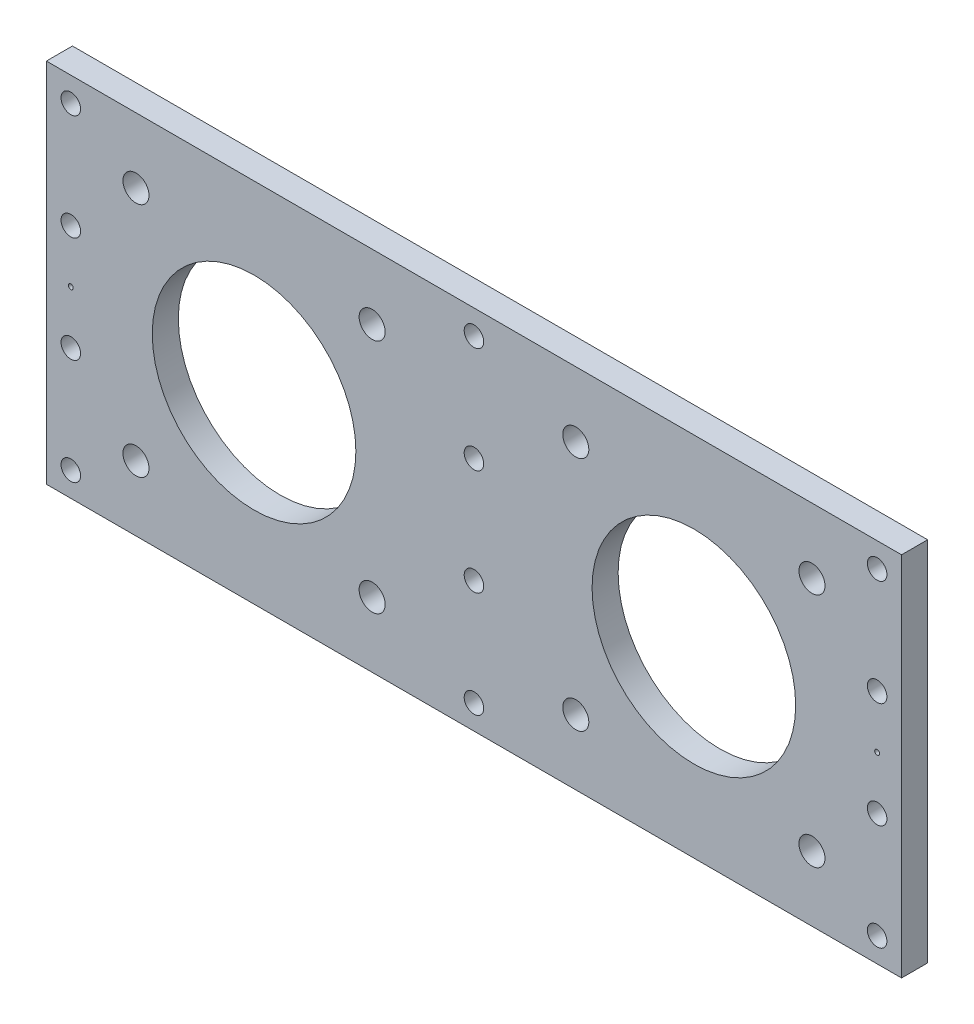
SolidWorks part; units mm, degrees
ref_plane "Front" through (0, 0, 0) normal (0, 0, 1) x (1, 0, 0)
ref_plane "Top" through (0, 0, 0) normal (0, 1, 0) x (1, 0, 0)
ref_plane "Right" through (0, 0, 0) normal (1, 0, 0) x (0, 0, -1)
sketch "Sketch1" plane through (0, 0, 0) normal (0, 0, 1) x (1, 0, 0)
  line L1 (-73.9828, 395.0592) -> (976.0172, 395.0592)
  line L2 (-73.9828, 395.0592) -> (-73.9828, -54.9408)
  line L3 (-73.9828, -54.9408) -> (976.0172, -54.9408)
  line L4 (976.0172, 395.0592) -> (976.0172, -54.9408)
extrude "Boss-Extrude1" add sketch "Sketch1" along normal blind 32
sketch "Sketch2" plane through (0, 0, 32) normal (0, 0, 1) x (1, 0, 0)
  line L0 (451.0172, 395.0592) -> (451.0172, -54.9408) construction
  line L1 (976.0172, 395.0592) -> (-73.9828, 395.0592) construction
  line L2 (-73.9828, -54.9408) -> (976.0172, -54.9408) construction
  line L3 (181.0172, 395.0592) -> (181.0172, -54.9408) construction
  line L4 (-73.9828, 170.0592) -> (976.0172, 170.0592) construction
  line L5 (-73.9828, 395.0592) -> (-73.9828, -54.9408) construction
  line L6 (976.0172, -54.9408) -> (976.0172, 395.0592) construction
  line L7 (721.0172, 395.0592) -> (721.0172, -54.9408) construction
  circle A0 centre (181.0172, 170.0592) radius 125
  circle A1 centre (721.0172, 170.0592) radius 125
  dimension "D2" = 125
  dimension "D3" = 125
  dimension "D1" = 255
extrude "Cut-Extrude1" cut sketch "Sketch2" against normal blind 32
sketch "Sketch3" plane through (0, 0, 32) normal (0, 0, 1) x (1, 0, 0)
  line L0 (976.0172, 395.0592) -> (-73.9828, 395.0592) construction
  line L1 (-73.9828, 395.0592) -> (-73.9828, -54.9408) construction
  line L2 (451.0172, 395.0592) -> (451.0172, -54.9408) construction
  line L3 (-73.9828, -54.9408) -> (976.0172, -54.9408) construction
  circle A0 centre (-43.9828, 365.0592) radius 12
  circle A1 centre (-43.9828, 235.0592) radius 12
  circle A2 centre (-43.9828, 105.0592) radius 12
  circle A3 centre (-43.9828, -24.9408) radius 12
  circle A4 centre (946.0172, -24.9408) radius 12
  circle A5 centre (946.0172, 105.0592) radius 12
  circle A6 centre (946.0172, 235.0592) radius 12
  circle A7 centre (946.0172, 365.0592) radius 12
  circle A8 centre (451.0172, 365.0592) radius 12
  circle A9 centre (451.0172, 235.0592) radius 12
  circle A10 centre (451.0172, 105.0592) radius 12
  circle A11 centre (451.0172, -24.9408) radius 12
  dimension "D1" = 24
  dimension "D2" = 30
  dimension "D3" = 30
  dimension "D5" = 12
  dimension "D4" = 4
  dimension "D6" = 4
extrude "Cut-Extrude2" cut sketch "Sketch3" against normal blind 32
sketch "Sketch4" plane through (0, 0, 32) normal (0, 0, 1) x (1, 0, 0)
  line L0 (181.0172, 295.0592) -> (181.0172, 45.0592) construction
  line L1 (181.0172, 170.0592) -> (36.0603, 315.0161) construction
  line L5 (56.0172, 170.0592) -> (306.0172, 170.0592) construction
  circle A0 centre (181.0172, 170.0592) radius 125 construction
  circle A1 centre (36.0603, 315.0161) radius 18
  circle A2 centre (181.0172, 170.0592) radius 205 construction
  dimension "D5" = 410
  dimension "D1" = 45
hole_wizard "M36 Tapped Hole1" positions "Sketch6" profile "Sketch5" tap size "M36" standard "GB"
sketch "Sketch6" plane through (0, 0, 32) normal (0, 0, 1) x (1, 0, 0)
  line L0 (181.0172, 170.0592) -> (36.0172, 315.0592) construction
  line L2 (181.0172, 170.0592) -> (181.0172, 495.7981) construction
  circle A1 centre (181.0172, 170.0592) radius 205.061 construction
  point P0 (36.0172, 315.0592)
  dimension "D1" = 410.1219
  dimension "D2" = 45
sketch "Sketch5" plane through (36.0172, 315.0592, 32) normal (1, 0, 0) x (0, -1, 0)
  line L0 (0, 0) -> (0, 101.6138)
  line L1 (0, 101.6138) -> (16, 92)
  line L2 (16, 92) -> (16, 0)
  line L5 (16, 0) -> (0, 0)
  line L10 (0, 101.6138) -> (-16, 92) construction
  line L11 (0, -6.35) -> (0, 107.95) construction
  dimension "螺纹孔钻头直径" = 32
  dimension "螺纹孔钻头深度" = 92
  dimension "导头角度" = 118
cosmetic thread "Cosmetic Thread4" parameters "D1"=32, "D2"=36
ref_plane "Plane1" through (451.0172, 0, 0) normal (-1, 0, 0) x (0, 0, 1)
mirror "Mirror1" about plane through (451.0172, 0, 0) normal (-1, 0, 0) of "M36 Tapped Hole1"
sketch "Sketch7" plane through (0, 0, 32) normal (0, 0, 1) x (1, 0, 0)
  line L0 (56.0172, 170.0592) -> (-73.9828, 170.0592) construction
  line L1 (-73.9828, 395.0592) -> (-73.9828, -54.9408) construction
  line L2 (-43.9828, 223.0592) -> (-43.9828, 117.0592) construction
  circle A0 centre (-43.9828, 235.0592) radius 12 construction
  circle A1 centre (-43.9828, 105.0592) radius 12 construction
  circle A2 centre (-43.9828, 170.0592) radius 3
  dimension "D1" = 3
extrude "Cut-Extrude3" cut sketch "Sketch7" against normal blind 32
mirror "Mirror2" about plane through (451.0172, 0, 0) normal (-1, 0, 0) of "Cut-Extrude3"
pattern_circular "CirPattern1" count 4 over 360 about axis through (181.0172, 170.0592, 0) along (0, 0, 1) of "M36 Tapped Hole1"
mirror "Mirror3" about plane through (451.0172, 0, 0) normal (-1, 0, 0) of "CirPattern1", "M36 Tapped Hole1"
equation "\"零件重量\"= IIF ( \"SW-质量\" > 100 , int ( \"SW-质量\" ) , \"SW-质量\" )"
